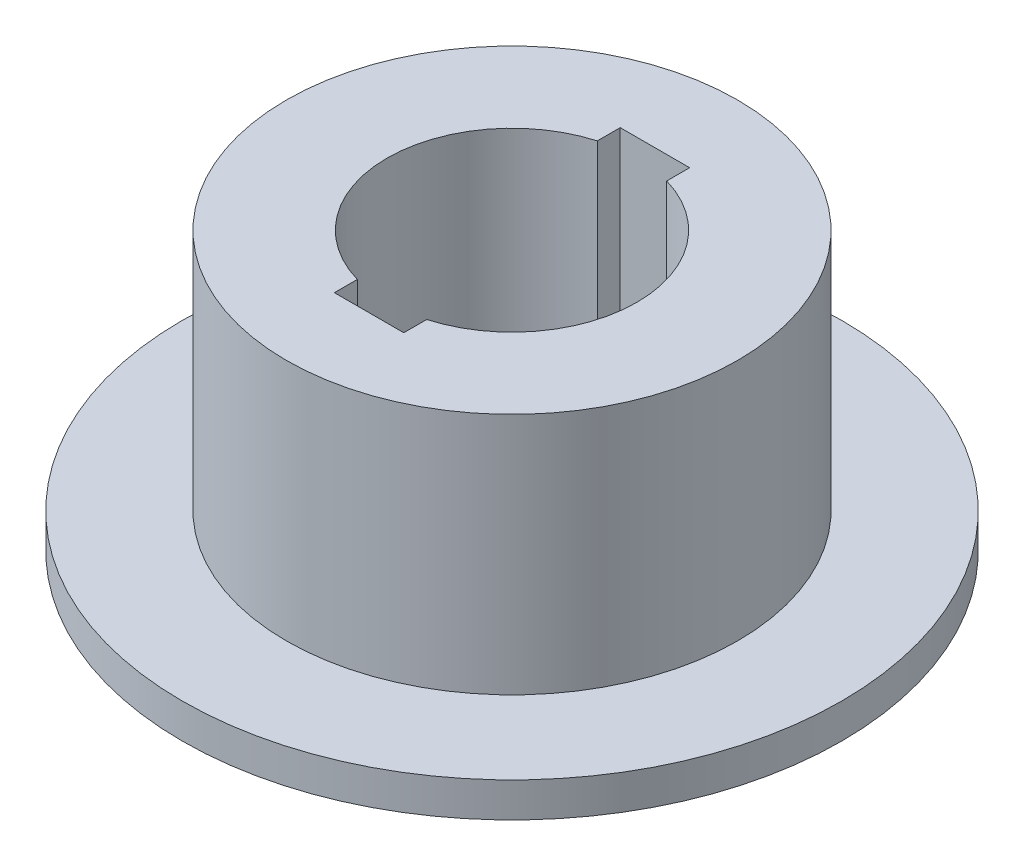
SolidWorks part; units mm, degrees
ref_plane "前视基准面" through (0, 0, 0) normal (0, 0, 1) x (1, 0, 0)
ref_plane "上视基准面" through (0, 0, 0) normal (0, 1, 0) x (1, 0, 0)
ref_plane "右视基准面" through (0, 0, 0) normal (1, 0, 0) x (0, 0, -1)
sketch "草图1" plane through (0, 0, 0) normal (0, 1, 0) x (1, 0, 0)
  line L0 (-37.1309, 0) -> (37.006, 0) construction
  line L1 (0, 20.5916) -> (5, 20.5916)
  line L2 (5, 20.5916) -> (5, 17.2916)
  line L3 (5, -20.5916) -> (5, -17.2916)
  line L4 (-5, 17.2916) -> (-5, 20.5916)
  line L5 (-5, 20.5916) -> (0, 20.5916)
  line L6 (0, -20.5916) -> (5, -20.5916)
  line L7 (-5, -20.5916) -> (0, -20.5916)
  line L8 (-5, -17.2916) -> (-5, -20.5916)
  arc A0 (-5, 17.2916) -> (-5, -17.2916) centre (0, 0) ccw
  circle A1 centre (0, 0) radius 32.5001
  arc A2 (5, -17.2916) -> (5, 17.2916) centre (0, 0) ccw
  dimension "D1" = 3.3
extrude "凸台-拉伸1" add sketch "草图1" along normal blind 40
sketch "草图2" plane through (0, 0, 0) normal (0, -1, 0) x (1, 0, 0)
  circle A0 centre (0, 0) radius 32.5
  circle A1 centre (0, 0) radius 47.5
extrude "凸台-拉伸2" add sketch "草图2" against normal blind 5
